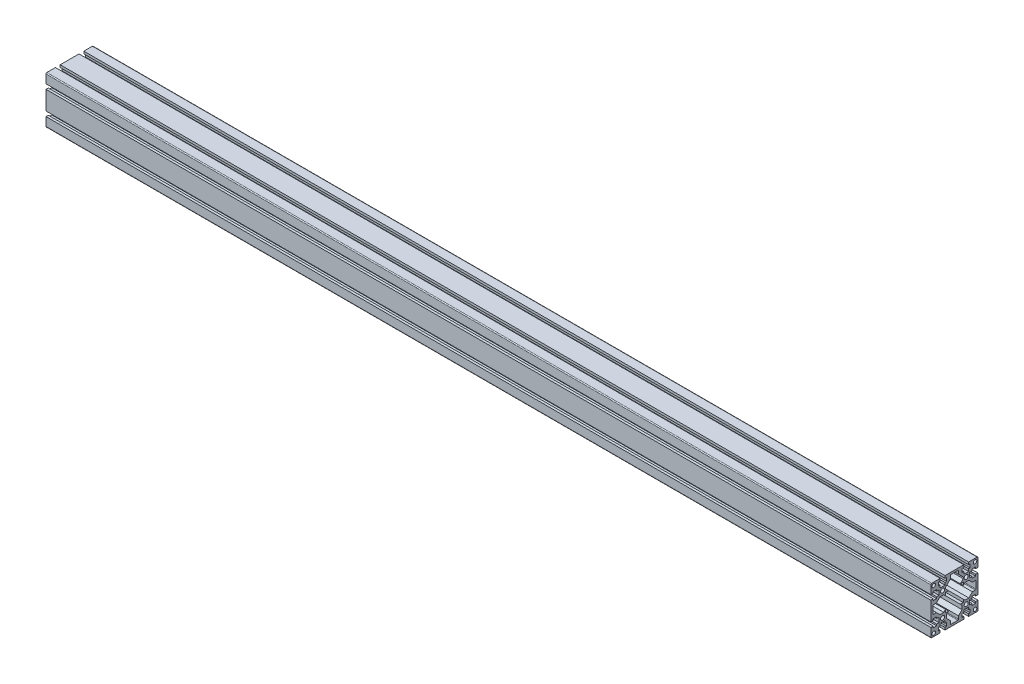
SolidWorks part; units mm, degrees
ref_plane "Front Plane" through (0, 0, 0) normal (0, 0, 1) x (1, 0, 0)
ref_plane "Top Plane" through (0, 0, 0) normal (0, 1, 0) x (1, 0, 0)
ref_plane "Right Plane" through (0, 0, 0) normal (1, 0, 0) x (0, 0, -1)
sketch "草图1" plane through (0, 0, 0) normal (0, 0, 1) x (1, 0, 0)
  line L0 (-530.3448, 0) -> (969.6552, 0)
  dimension "D1" = 1500
other "Aluminium profile 80 X 80G X R1.5(1)"
ref_plane "Plane2" through (-530.3448, 0, 0) normal (1, 0, 0) x (0, 1, 0)
sketch "Sketch1" plane through (-530.3448, 0, 0) normal (1, 0, 0) x (0, 1, 0)
  line L0 (0, 40) -> (0, 0) construction
  line L1 (0, 0) -> (40, 0) construction
  line L2 (-24.05, 40) -> (-24.05, 36)
  line L3 (-38.5, 40) -> (-24.05, 40)
  line L4 (-40, 38.5) -> (-40, 24.05)
  line L5 (-38.5, -40) -> (-24.05, -40)
  line L6 (40, 38.5) -> (40, 24.05)
  line L7 (-24.05, 36) -> (-26.75, 36)
  line L8 (-26.75, 36) -> (-26.75, 30)
  line L9 (-26.75, 30) -> (-24.05, 30)
  line L10 (-24.05, 30) -> (-24.05, 26)
  line L11 (-24.05, 26) -> (-15.95, 26)
  line L12 (-15.95, 26) -> (-15.95, 30)
  line L13 (-15.95, 30) -> (-13.25, 30)
  line L14 (-13.25, 30) -> (-13.25, 36)
  line L15 (-13.25, 36) -> (-15.95, 36)
  line L16 (-15.95, 36) -> (-15.95, 40)
  line L17 (-40, 15.95) -> (-36, 15.95)
  line L18 (-36, 15.95) -> (-36, 13.25)
  line L19 (-15.95, 40) -> (15.95, 40)
  line L20 (-20, 20) -> (-20, 40) construction
  line L21 (20, 20) -> (20, 40) construction
  line L22 (15.95, 36) -> (15.95, 40)
  line L23 (13.25, 36) -> (15.95, 36)
  line L24 (13.25, 30) -> (13.25, 36)
  line L25 (15.95, 30) -> (13.25, 30)
  line L26 (-36, 13.25) -> (-30, 13.25)
  line L27 (-30, 13.25) -> (-30, 15.95)
  line L28 (-26, 15.95) -> (-26, 24.05)
  line L29 (-26, 24.05) -> (-30, 24.05)
  line L30 (-30, 24.05) -> (-30, 26.75)
  line L31 (-30, 26.75) -> (-36, 26.75)
  line L32 (-36, 26.75) -> (-36, 24.05)
  line L33 (-36, 24.05) -> (-40, 24.05)
  line L34 (-30, 15.95) -> (-26, 15.95)
  line L35 (15.95, 26) -> (15.95, 30)
  line L36 (24.05, 26) -> (15.95, 26)
  line L37 (24.05, 30) -> (24.05, 26)
  line L38 (26.75, 30) -> (24.05, 30)
  line L39 (26.75, 36) -> (26.75, 30)
  line L40 (24.05, 36) -> (26.75, 36)
  line L41 (24.05, 40) -> (24.05, 36)
  line L42 (24.05, -40) -> (24.05, -36)
  line L43 (24.05, -36) -> (26.75, -36)
  line L44 (26.75, -36) -> (26.75, -30)
  line L45 (26.75, -30) -> (24.05, -30)
  line L46 (24.05, -30) -> (24.05, -26)
  line L47 (24.05, -26) -> (15.95, -26)
  line L48 (15.95, -26) -> (15.95, -30)
  line L49 (15.95, -30) -> (13.25, -30)
  line L50 (13.25, -30) -> (13.25, -36)
  line L51 (13.25, -36) -> (15.95, -36)
  line L52 (15.95, -36) -> (15.95, -40)
  line L53 (-15.95, -36) -> (-15.95, -40)
  line L54 (-13.25, -36) -> (-15.95, -36)
  line L55 (-13.25, -30) -> (-13.25, -36)
  line L56 (-15.95, -30) -> (-13.25, -30)
  line L57 (-15.95, -26) -> (-15.95, -30)
  line L58 (-24.05, -26) -> (-15.95, -26)
  line L59 (-24.05, -30) -> (-24.05, -26)
  line L60 (-26.75, -30) -> (-24.05, -30)
  line L61 (-26.75, -36) -> (-26.75, -30)
  line L62 (-24.05, -36) -> (-26.75, -36)
  line L63 (-24.05, -40) -> (-24.05, -36)
  line L64 (-30, -15.95) -> (-26, -15.95)
  line L65 (-36, -26.75) -> (-36, -24.05)
  line L66 (-30, -26.75) -> (-36, -26.75)
  line L67 (-30, -24.05) -> (-30, -26.75)
  line L68 (-26, -24.05) -> (-30, -24.05)
  line L69 (-26, -15.95) -> (-26, -24.05)
  line L70 (-30, -13.25) -> (-30, -15.95)
  line L71 (-36, -13.25) -> (-30, -13.25)
  line L72 (-36, -15.95) -> (-36, -13.25)
  line L73 (36, 24.05) -> (40, 24.05)
  line L74 (40, 15.95) -> (36, 15.95)
  line L75 (36, -15.95) -> (36, -13.25)
  line L76 (36, -13.25) -> (30, -13.25)
  line L77 (30, -13.25) -> (30, -15.95)
  line L78 (26, -15.95) -> (26, -24.05)
  line L79 (26, -24.05) -> (30, -24.05)
  line L80 (30, -24.05) -> (30, -26.75)
  line L81 (30, -26.75) -> (36, -26.75)
  line L82 (36, -26.75) -> (36, -24.05)
  line L83 (30, -15.95) -> (26, -15.95)
  line L84 (30, 15.95) -> (26, 15.95)
  line L85 (36, 26.75) -> (36, 24.05)
  line L86 (30, 26.75) -> (36, 26.75)
  line L87 (30, 24.05) -> (30, 26.75)
  line L88 (26, 24.05) -> (30, 24.05)
  line L89 (26, 15.95) -> (26, 24.05)
  line L90 (30, 13.25) -> (30, 15.95)
  line L91 (36, 13.25) -> (30, 13.25)
  line L92 (36, 15.95) -> (36, 13.25)
  line L93 (-36, -15.95) -> (-40, -15.95)
  line L94 (-36, -24.05) -> (-40, -24.05)
  line L95 (36, -15.95) -> (40, -15.95)
  line L96 (36, -24.05) -> (40, -24.05)
  line L97 (-13, 18) -> (-10, 15)
  line L98 (-15, 15) -> (-10, 15)
  line L99 (-15, 15) -> (-15, 10)
  line L100 (-15, -15) -> (-10, -15)
  line L101 (15, 15) -> (15, 10)
  line L102 (-18, 13) -> (-15, 10)
  line L104 (13, 18) -> (10, 15)
  line L105 (13, -18) -> (10, -15)
  line L106 (20, -15) -> (15, -10)
  line L107 (-18, -13) -> (-15, -10)
  line L108 (-13, -18) -> (-10, -15)
  line L109 (15, -10) -> (15, -15)
  line L110 (10, 15) -> (15, 15)
  line L111 (-15, -10) -> (-15, -15)
  line L112 (10, -15) -> (15, -15)
  line L113 (15, 10) -> (20, 15)
  line L235 (24.05, 40) -> (38.5, 40)
  line L249 (-40, 15.95) -> (-40, -15.95)
  line L250 (-20, 20) -> (-26, 20) construction
  line L264 (40, 15.95) -> (40, -15.95)
  line L265 (-13, 24.5) -> (-7, 30.5)
  line L266 (-7, 30.5) -> (-7, 35.5)
  line L267 (7, 35.5) -> (7, 30.5)
  line L268 (7, 30.5) -> (13, 24.5)
  line L269 (-6, -36.5) -> (6, -36.5)
  line L270 (-13, 24.5) -> (-13, 18)
  line L271 (-35.5, 7) -> (-30.5, 7)
  line L272 (-30.5, 7) -> (-24.5, 13)
  line L273 (-24.5, 13) -> (-18, 13)
  line L274 (13, 24.5) -> (13, 18)
  line L275 (-15.95, -40) -> (15.95, -40)
  line L276 (35.5, 7) -> (30.5, 7)
  line L277 (30.5, 7) -> (22.5, 15)
  line L278 (24.05, -40) -> (38.5, -40)
  line L279 (20, 15) -> (22.5, 15)
  line L333 (-13, -24.5) -> (-13, -18)
  line L336 (-13, -24.5) -> (-7, -30.5)
  line L385 (-7, -30.5) -> (-7, -35.5)
  line L386 (-36.5, 6) -> (-36.5, -6)
  line L387 (7, -35.5) -> (7, -30.5)
  line L429 (7, -30.5) -> (13, -24.5)
  line L430 (13, -24.5) -> (13, -18)
  line L494 (20, -15) -> (22.5, -15)
  line L496 (30.5, -7) -> (22.5, -15)
  line L497 (35.5, -7) -> (30.5, -7)
  line L498 (-24.5, -13) -> (-18, -13)
  line L499 (-30.5, -7) -> (-24.5, -13)
  line L500 (-35.5, -7) -> (-30.5, -7)
  line L512 (40, -24.05) -> (40, -38.5)
  line L519 (-40, -24.05) -> (-40, -38.5)
  line L520 (-6, 36.5) -> (6, 36.5)
  line L523 (36.5, 6) -> (36.5, -6)
  circle A0 centre (-20, 20) radius 3.4
  circle A2 centre (20, 20) radius 3.4
  circle A3 centre (20, -20) radius 3.4
  circle A7 centre (-20, -20) radius 3.4
  arc A8 (-38.5, 40) -> (-40, 38.5) centre (-38.5, 38.5) ccw
  arc A9 (-40, -38.5) -> (-38.5, -40) centre (-38.5, -38.5) ccw
  arc A10 (38.5, -40) -> (40, -38.5) centre (38.5, -38.5) ccw
  arc A11 (38.5, 40) -> (40, 38.5) centre (38.5, 38.5) cw
  circle A12 centre (-35, 35) radius 3
  circle A13 centre (35, 35) radius 3
  circle A14 centre (35, -35) radius 3
  arc A15 (-6, 36.5) -> (-7, 35.5) centre (-6, 35.5) ccw
  arc A16 (6, 36.5) -> (7, 35.5) centre (6, 35.5) cw
  arc A17 (-36.5, 6) -> (-35.5, 7) centre (-35.5, 6) cw
  arc A18 (-36.5, -6) -> (-35.5, -7) centre (-35.5, -6) ccw
  arc A19 (36.5, -6) -> (35.5, -7) centre (35.5, -6) cw
  arc A20 (36.5, 6) -> (35.5, 7) centre (35.5, 6) ccw
  arc A21 (6, -36.5) -> (7, -35.5) centre (6, -35.5) ccw
  arc A22 (-6, -36.5) -> (-7, -35.5) centre (-6, -35.5) cw
  point P48 (-20, 20)
  point P97 (0, 0)
  point P104 (-7, 36.5)
  point P185 (40, 40)
  point P187 (40, -40)
  point P188 (-40, -40)
  point P190 (-40, 40)
  dimension "D1" = 80
  dimension "D2" = 80
  dimension "D3" = 20
  dimension "D4" = 8.1
  dimension "D5" = 45
  dimension "D6" = 7
  dimension "D7" = 13.5
  dimension "D8" = 6
  dimension "D12" = 5
  dimension "D13" = 5
  dimension "D14" = 20
  dimension "D18" = 1
  dimension "D19" = 14
  dimension "D15" = 6.8
  dimension "D27" = 45
  dimension "D20" = 1.5
  dimension "D11" = 6
  dimension "D9" = 4
  dimension "D10" = 14
  dimension "D16" = 14
  dimension "D17" = 45
  dimension "D21" = 3.5
  dimension "D22" = 3.5
  dimension "D23" = 73
  dimension "D24" = 30
  dimension "D25" = 30
  dimension "D26" = 45
  dimension "D28" = 5
sketch "Sketch10" plane through (969.6552, 0, 0) normal (1, 0, 0) x (0, 0, -1)
  circle A0 centre (35, -35) radius 3
  circle A1 centre (-35, -35) radius 3 construction
  circle A2 centre (35, 35) radius 3 construction
  dimension "D1" = 6
  dimension "D2" = 70
  dimension "D3" = 70
extrude "Cut-Extrude1" cut sketch "Sketch10" against normal through all
